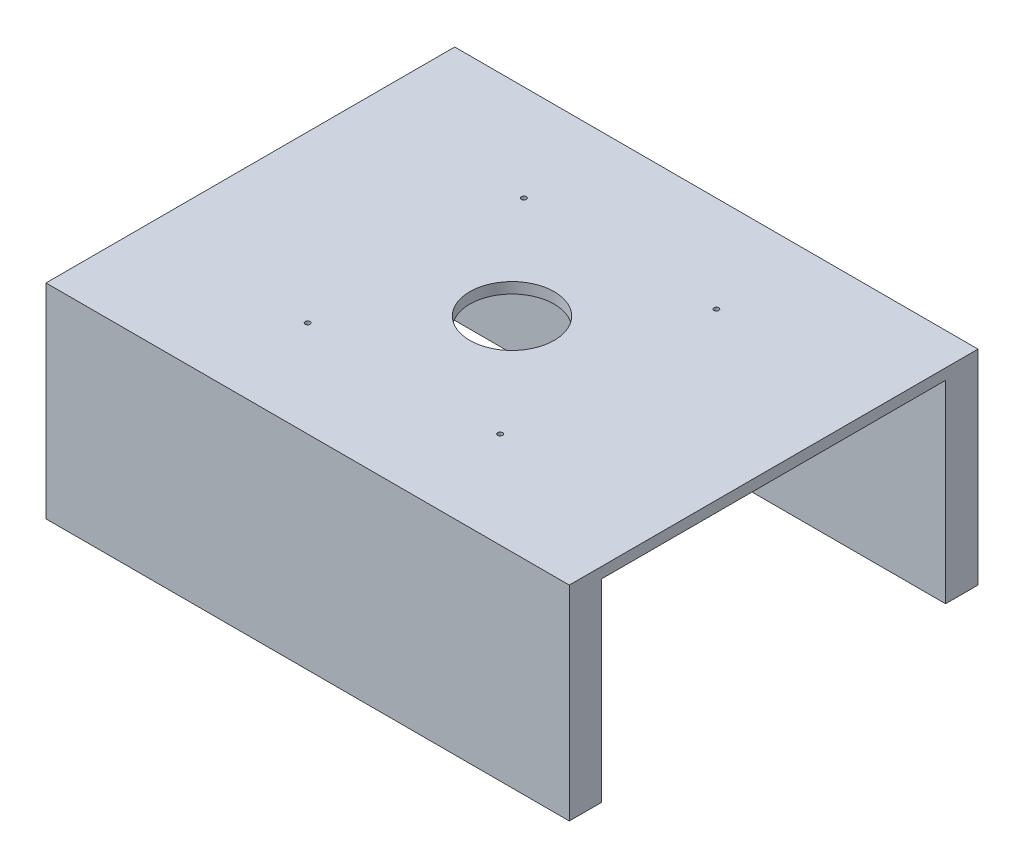
from build123d import *

# Parameters (mm, degrees)
SKETCH1_W           = 484
SKETCH1_H           = 378
BOSS_EXTRUDE1_DEPTH = 189
SKETCH2_W           = 318
SKETCH2_H           = 179
CUT_EXTRUDE1_DEPTH  = 553.899629228
SKETCH3_R           = 2.25
SKETCH3_R_2         = 39.056616246
CUT_EXTRUDE2_DEPTH  = 361.563447953


with BuildPart() as part:
    # Sketch1 → Boss-Extrude1 (new body)
    with BuildSketch(Plane(origin=(0, 0, 0), x_dir=(1, 0, 0), z_dir=(0, 1, 0))):
        Rectangle(SKETCH1_W, SKETCH1_H)
    extrude(amount=BOSS_EXTRUDE1_DEPTH)

    # Sketch2 → Cut-Extrude1 (cut, through all)
    with BuildSketch(Plane.ZY.offset(242)):
        with Locations((0, 89.5)):
            Rectangle(SKETCH2_W, SKETCH2_H)
    extrude(amount=-CUT_EXTRUDE1_DEPTH, mode=Mode.SUBTRACT)

    # Sketch3 → Cut-Extrude2 (cut, through all)
    with BuildSketch(Plane(origin=(0, 189, 0), x_dir=(1, 0, 0), z_dir=(0, 1, 0))):
        with Locations(Location((-89, -100, 0), (0, 0, 270))):
            Circle(SKETCH3_R)
        with Locations(Location((89, -100, 0), (0, 0, 270))):
            Circle(SKETCH3_R)
        with Locations(Location((-89, 100, 0), (0, 0, 270))):
            Circle(SKETCH3_R)
        with Locations(Location((89, 100, 0), (0, 0, 270))):
            Circle(SKETCH3_R)
        with Locations(Location((0, 0, 0), (0, 0, 270))):
            Circle(SKETCH3_R_2)
    extrude(amount=-CUT_EXTRUDE2_DEPTH, mode=Mode.SUBTRACT)


solid = part.part
